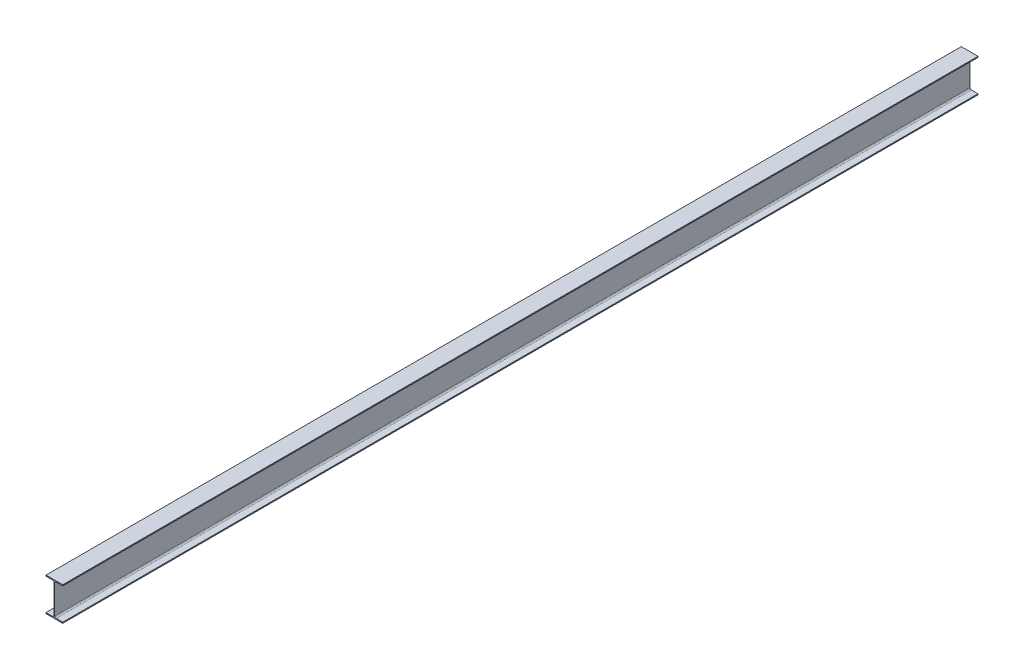
from build123d import *

# Parameters (mm, degrees)
BOSS_EXTRUDE1_DEPTH = 8210


with BuildPart() as part:
    # Sketch1 → Boss-Extrude1 (new body)
    with BuildSketch(Plane.XY):
        with BuildLine():
            Line((75, 0), (-75, 0))
            Line((-75, 0), (-75, 9))
            Line((-75, 9), (-16.25, 9))
            ThreePointArc((-16.25, 9), (-7.057611845, 12.807611845), (-3.25, 22))
            Line((-3.25, 22), (-3.25, 278))
            ThreePointArc((-3.25, 278), (-7.057611845, 287.192388155), (-16.25, 291))
            Line((-16.25, 291), (-75, 291))
            Line((-75, 291), (-75, 300))
            Line((-75, 300), (75, 300))
            Line((75, 300), (75, 291))
            Line((75, 291), (16.25, 291))
            ThreePointArc((16.25, 291), (7.057611845, 287.192388155), (3.25, 278))
            Line((3.25, 278), (3.25, 22))
            ThreePointArc((3.25, 22), (7.057611845, 12.807611845), (16.25, 9))
            Line((16.25, 9), (75, 9))
            Line((75, 9), (75, 0))
        make_face()
    extrude(amount=BOSS_EXTRUDE1_DEPTH)


solid = part.part
